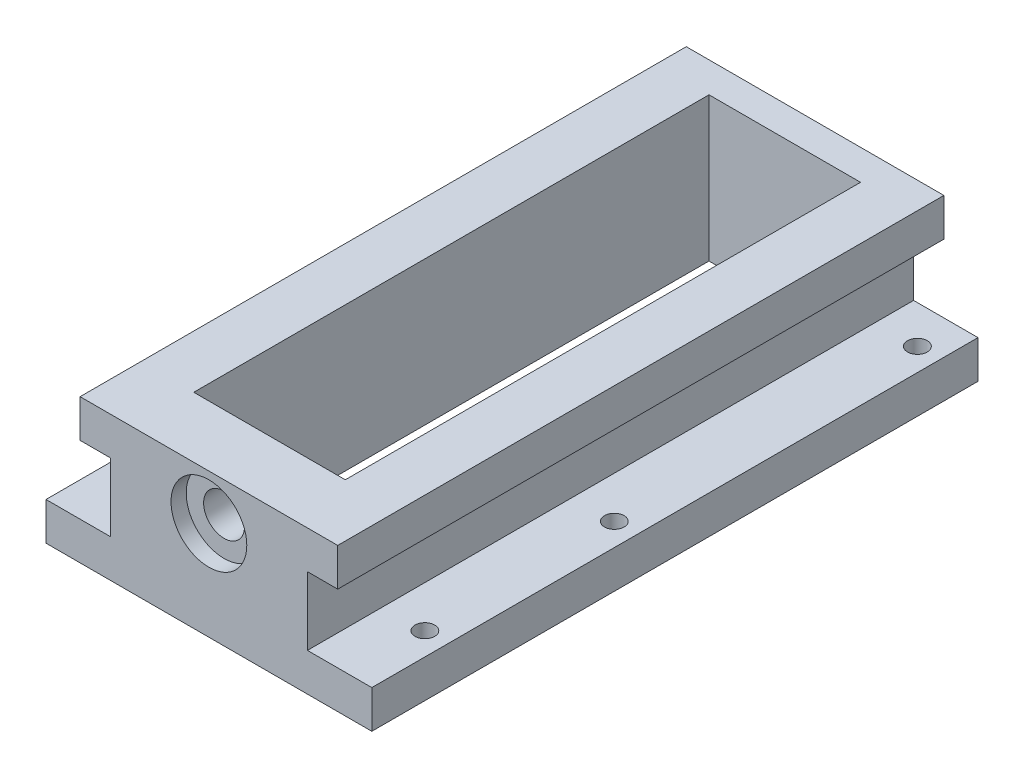
from build123d import *

# Parameters (mm, degrees)
EXTRUDE_1_DEPTH             = 400
CUT_EXTRUDE_1_REACH         = 426.949
SKETCH_2_W                  = 100
SKETCH_2_H                  = 340
CUT_EXTRUDE_2_REACH         = 426.949
SKETCH_3_R                  = 13.5
SKETCH_4_R                  = 25
CUT_EXTRUDE_3_DEPTH         = 10
CUT_EXTRUDE_START           = -30
SKETCH_4_2_R                = 25
CUT_EXTRUDE_4_DEPTH         = 10
HOLE_WIZARD_13_0_13_1_D     = 13
HOLE_WIZARD_13_0_13_1_DEPTH = 70
HOLE_WIZARD_13_0_13_1_TIP   = 3.905594024


with BuildPart() as part:
    # 草图1 → 凸台-拉伸1 (new body)
    with BuildSketch(Plane.XY):
        Polygon((-107.5, 0), (107.5, 0), (107.5, 25), (65, 25), (65, 70), (85, 70), (85, 95), (-85, 95), (-85, 70), (-65, 70), (-65, 25), (-107.5, 25), align=None)
    extrude(amount=EXTRUDE_1_DEPTH)

    # 草图2 → 切除-拉伸1 (cut, up to next)
    with BuildSketch(Plane(origin=(0, 95, 0), x_dir=(1, 0, 0), z_dir=(0, 1, 0)), mode=Mode.PRIVATE) as cut_extrude_1_sk1:
        with Locations((0, -190)):
            Rectangle(SKETCH_2_W, SKETCH_2_H)
    cut_extrude_1_tool1 = extrude(cut_extrude_1_sk1.sketch, amount=-CUT_EXTRUDE_1_REACH, mode=Mode.PRIVATE) & part.part
    add(cut_extrude_1_tool1.solids().sort_by_distance((0, 95, 190))[0], mode=Mode.SUBTRACT)

    # 草图3 → 切除-拉伸2 (cut, up to next)
    with BuildSketch(Plane.XY.offset(400), mode=Mode.PRIVATE) as cut_extrude_2_sk1:
        with Locations((0, 65)):
            Circle(SKETCH_3_R)
    cut_extrude_2_tool1 = extrude(cut_extrude_2_sk1.sketch, amount=-CUT_EXTRUDE_2_REACH, mode=Mode.PRIVATE) & part.part
    add(cut_extrude_2_tool1.solids().sort_by_distance((0, 65, 400))[0], mode=Mode.SUBTRACT)

    # 草图4 → 切除-拉伸3 (cut)
    with BuildSketch(Plane.XY.offset(400)):
        with Locations((0, 65)):
            Circle(SKETCH_4_R)
    extrude(amount=-CUT_EXTRUDE_3_DEPTH, mode=Mode.SUBTRACT)

    # 草图4<2> → 切除-拉伸4 (cut)
    with BuildSketch(Plane.XY.offset(400).offset(CUT_EXTRUDE_START)):
        with Locations((0, 65)):
            Circle(SKETCH_4_2_R)
    extrude(amount=-CUT_EXTRUDE_4_DEPTH, mode=Mode.SUBTRACT)

    # Ø13.0 (13) 直径孔1
    with Locations(Plane(origin=(0, 25, 0), x_dir=(1, 0, 0), z_dir=(0, 1, 0))):
        with Locations((-92.5, -350), (92.5, -350), (-92.5, -225), (92.5, -225), (-92.5, -25), (92.5, -25)):
            Hole(HOLE_WIZARD_13_0_13_1_D / 2, depth=HOLE_WIZARD_13_0_13_1_DEPTH)
            with Locations((0, 0, -(HOLE_WIZARD_13_0_13_1_DEPTH + HOLE_WIZARD_13_0_13_1_TIP / 2))):  # 118° drill point
                Cone(0, HOLE_WIZARD_13_0_13_1_D / 2, HOLE_WIZARD_13_0_13_1_TIP, mode=Mode.SUBTRACT)


solid = part.part
